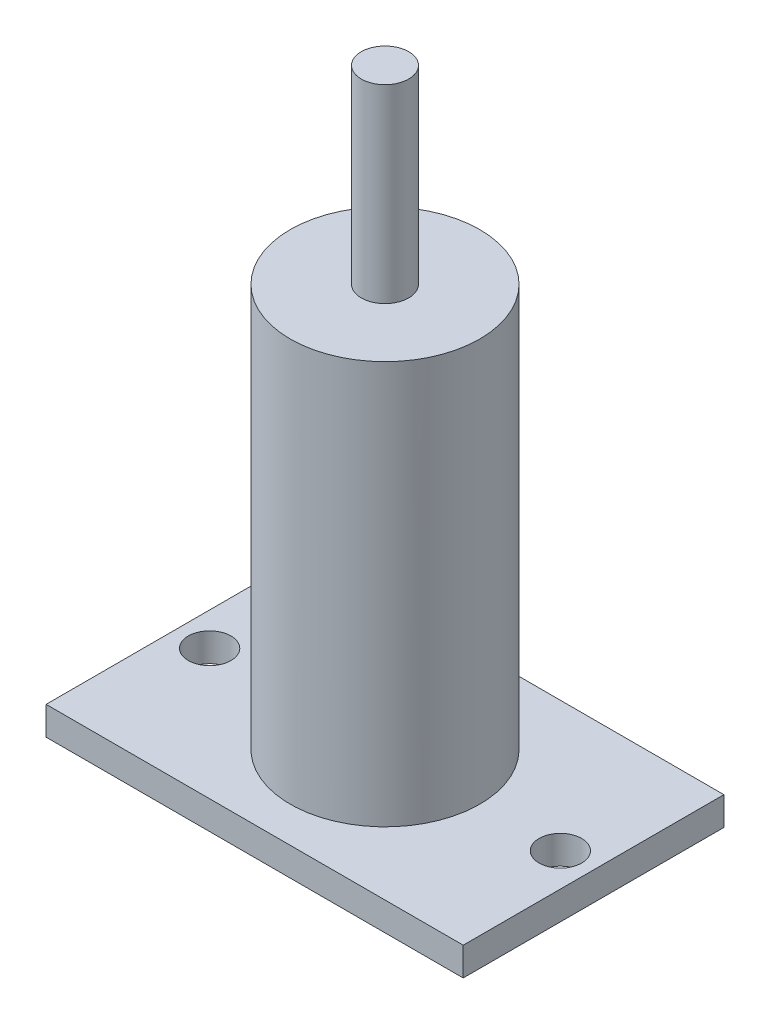
SolidWorks part; units mm, degrees
material "标准件"
ref_plane "前视基准面" through (0, 0, 0) normal (0, 0, 1) x (1, 0, 0)
ref_plane "上视基准面" through (0, 0, 0) normal (0, 1, 0) x (1, 0, 0)
ref_plane "右视基准面" through (0, 0, 0) normal (1, 0, 0) x (0, 0, -1)
sketch "草图1" plane through (0, 0, 0) normal (0, 1, 0) x (1, 0, 0)
  line L1 (-44, -27.5) -> (44, -27.5)
  line L2 (-44, -27.5) -> (-44, 27.5)
  line L3 (-44, 27.5) -> (44, 27.5)
  line L4 (44, -27.5) -> (44, 27.5)
  line L5 (-44, -27.5) -> (44, 27.5) construction
  line L6 (-44, 27.5) -> (44, -27.5) construction
  point P0 (0, 0)
  dimension "D1" = 88
  dimension "D2" = 55
extrude "凸台-拉伸1" add sketch "草图1" along normal blind 6
hole_wizard "M8 间隙孔1" positions "草图2" profile "草图3" hole size "M8" standard "ISO" end condition through all
sketch "草图2" plane through (0, 6, 0) normal (0, 1, 0) x (1, 0, 0)
  line L0 (0, 27.5) -> (0, -27.5) construction
  line L1 (44, 27.5) -> (-44, 27.5) construction
  line L2 (-44, -27.5) -> (44, -27.5) construction
  point P0 (-37, 0)
  point P2 (37, 0)
  dimension "D1" = 74
sketch "草图3" plane through (-37, 6, 0) normal (1, 0, 0) x (0, 0, 1)
  line L0 (0, 0) -> (0, 6)
  line L1 (0, 6) -> (4.5, 6)
  line L2 (4.5, 6) -> (4.5, 0)
  line L5 (4.5, 0) -> (0, 0)
  line L11 (0, -6.35) -> (0, 107.95) construction
  dimension "通孔孔直径" = 9
  dimension "通孔孔深度" = 6
sketch "草图4" plane through (0, 6, 0) normal (0, 1, 0) x (1, 0, 0)
  circle A0 centre (0, 0) radius 20
  dimension "D1" = 40
extrude "凸台-拉伸2" add sketch "草图4" along normal blind 85
sketch "草图5" plane through (0, 91, 0) normal (0, 1, 0) x (1, 0, 0)
  circle A0 centre (0, 0) radius 5
  dimension "D1" = 10
extrude "凸台-拉伸3" add sketch "草图5" along normal blind 40
